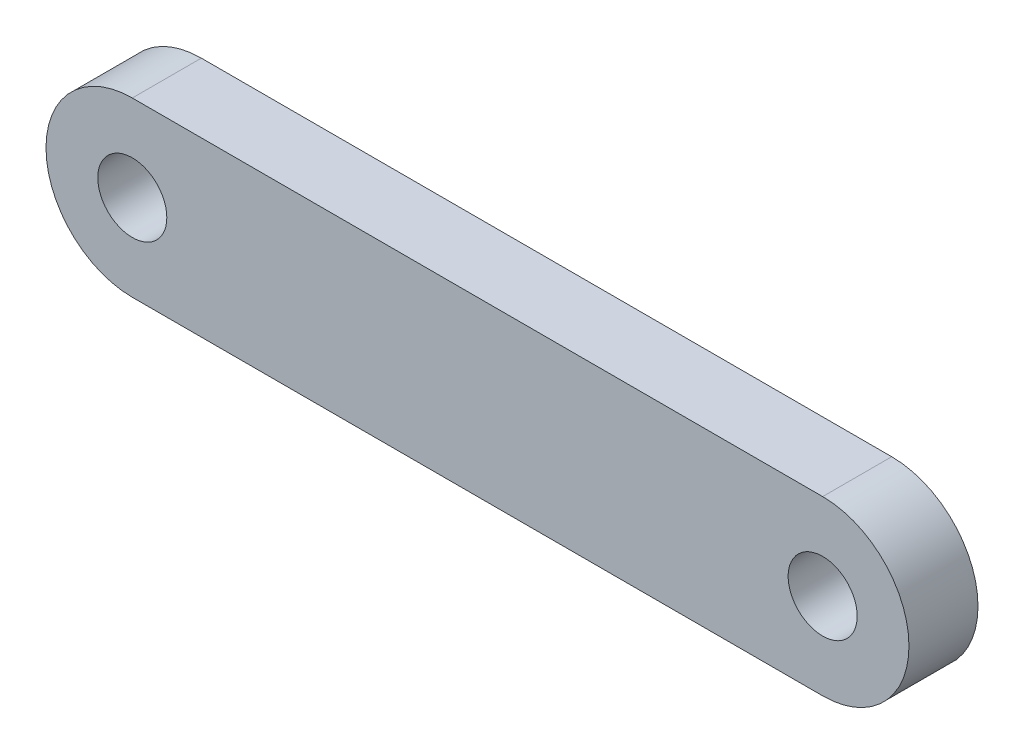
from build123d import *

# Parameters (mm, degrees)
SKETCH1_R           = 3
BOSS_EXTRUDE1_DEPTH = 6


with BuildPart() as part:
    # Sketch1 → Boss-Extrude1 (new body)
    with BuildSketch(Plane.XY):
        with BuildLine():
            Line((0, 7.5), (60, 7.5))
            ThreePointArc((60, 7.5), (67.5, 0), (60, -7.5))
            Line((60, -7.5), (0, -7.5))
            ThreePointArc((0, -7.5), (-7.5, 0), (0, 7.5))
        make_face()
        Circle(SKETCH1_R, mode=Mode.SUBTRACT)
        with Locations((60, 0)):
            Circle(SKETCH1_R, mode=Mode.SUBTRACT)
    extrude(amount=BOSS_EXTRUDE1_DEPTH)


solid = part.part
